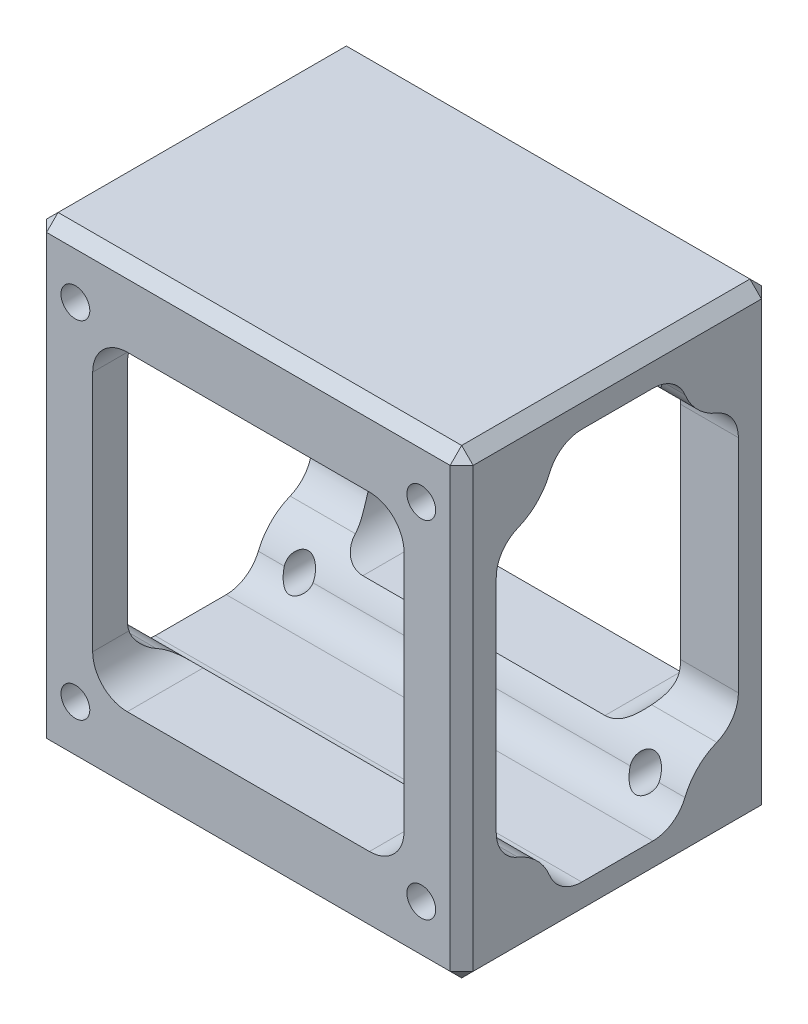
SolidWorks part; units mm, degrees
material "6061 合金"
ref_plane "前视基准面" through (0, 0, 0) normal (0, 0, 1) x (1, 0, 0)
ref_plane "上视基准面" through (0, 0, 0) normal (0, 1, 0) x (1, 0, 0)
ref_plane "右视基准面" through (0, 0, 0) normal (1, 0, 0) x (0, 0, -1)
other "Configuration Table"
sketch "草图1" plane through (0, 0, 0) normal (0, 1, 0) x (1, 0, 0)
  line L1 (-18.5, -13.5) -> (18.5, -13.5)
  line L2 (-18.5, -13.5) -> (-18.5, 13.5)
  line L3 (-18.5, 13.5) -> (18.5, 13.5)
  line L4 (18.5, -13.5) -> (18.5, 13.5)
  line L5 (-18.5, -13.5) -> (18.5, 13.5) construction
  line L6 (-18.5, 13.5) -> (18.5, -13.5) construction
  point P0 (0, 0)
  dimension "D1" = 27
  dimension "D2" = 37
extrude "凸台-拉伸1" add sketch "草图1" along normal blind 40
sketch "草图2" plane through (0, 40, 0) normal (0, 1, 0) x (1, 0, 0)
  line L1 (-10.5, -8.5) -> (10.5, -8.5)
  line L2 (-13.5, -5.5) -> (-13.5, 5.5)
  line L3 (-10.5, 8.5) -> (10.5, 8.5)
  line L4 (13.5, -5.5) -> (13.5, 5.5)
  line L5 (-13.5, -8.5) -> (13.5, 8.5) construction
  line L6 (-13.5, 8.5) -> (13.5, -8.5) construction
  line L14 (15.5, -10.5) -> (15.5, 10.5)
  line L15 (15.5, 10.5) -> (-15.5, 10.5)
  line L16 (-15.5, 10.5) -> (-15.5, -10.5)
  line L17 (-15.5, -10.5) -> (15.5, -10.5)
  line L18 (15.5, -10.5) -> (15.5, 10.5) construction
  line L19 (15.5, 10.5) -> (-15.5, 10.5) construction
  line L20 (-15.5, 10.5) -> (-15.5, -10.5) construction
  line L21 (-15.5, -10.5) -> (15.5, -10.5) construction
  arc A0 (10.5, -8.5) -> (13.5, -5.5) centre (10.5, -5.5) ccw
  arc A1 (-13.5, 5.5) -> (-10.5, 8.5) centre (-10.5, 5.5) cw
  arc A2 (-10.5, -8.5) -> (-13.5, -5.5) centre (-10.5, -5.5) cw
  arc A3 (10.5, 8.5) -> (13.5, 5.5) centre (10.5, 5.5) cw
  circle A4 centre (-15.5, 10.5) radius 1.25 construction
  circle A5 centre (15.5, 10.5) radius 1.25 construction
  circle A6 centre (15.5, -10.5) radius 1.25 construction
  circle A7 centre (-15.5, -10.5) radius 1.25 construction
  point P0 (0, 0)
  dimension "D1" = 17
  dimension "D3" = 3
  dimension "D5" = 2.5
  dimension "D2" = 27
  dimension "D4" = 3
extrude "切除-拉伸2" [suppressed] cut sketch "草图2" against normal through all
sketch "草图3" plane through (0, 0, -13.5) normal (0, 0, -1) x (-1, 0, 0)
  line L4 (18.5, 40) -> (18.5, 0) construction
  line L5 (-15, 5) -> (15, 5) construction
  line L6 (-15, 5) -> (-15, 35) construction
  line L7 (-15, 35) -> (15, 35) construction
  line L8 (15, 5) -> (15, 35) construction
  line L9 (18.5, 40) -> (18.5, 0) construction
  line L10 (-10.5, 6.5) -> (10.5, 6.5)
  line L11 (13.5, 9.5) -> (13.5, 30.5)
  line L12 (-10.5, 33.5) -> (10.5, 33.5)
  line L13 (-13.5, 9.5) -> (-13.5, 30.5)
  line L15 (-13.5, 33.5) -> (13.5, 33.5) construction
  line L16 (-13.5, 6.5) -> (-13.5, 33.5) construction
  line L17 (13.5, 6.5) -> (13.5, 33.5) construction
  line L18 (-13.5, 6.5) -> (13.5, 6.5) construction
  circle A0 centre (-15, 35) radius 1.25
  circle A1 centre (15, 35) radius 1.25
  circle A2 centre (-15, 5) radius 1.25
  circle A3 centre (15, 5) radius 1.25
  arc A4 (-10.5, 33.5) -> (-13.5, 30.5) centre (-10.5, 30.5) ccw
  arc A5 (13.5, 30.5) -> (10.5, 33.5) centre (10.5, 30.5) ccw
  arc A6 (10.5, 6.5) -> (13.5, 9.5) centre (10.5, 9.5) ccw
  arc A7 (-10.5, 6.5) -> (-13.5, 9.5) centre (-10.5, 9.5) cw
  point P4 (0, 5)
  point P7 (18.5, 20)
  point P8 (15, 20)
  dimension "D2" = 2.5
  dimension "D4" = 3
  dimension "D1" = 30
  dimension "D3" = 1.5
extrude "切除-拉伸3" cut sketch "草图3" against normal through all
hole_wizard "M3 螺纹孔1" positions "3D草图1" profile "草图6" tap size "M3" standard "GB" end condition through all
sketch3d "3D草图1"
  line L0 (-15, 5, 13.5) -> (-15, 5, -13.5) construction
  line L1 (-15, 35, 13.5) -> (-15, 35, -13.5) construction
  line L2 (15, 35, 13.5) -> (15, 35, -13.5) construction
  line L3 (15, 5, 13.5) -> (15, 5, -13.5) construction
  point P0 (-15, 5, -13.5)
  point P4 (-15, 35, -13.5)
  point P8 (15, 35, -13.5)
  point P12 (15, 5, -13.5)
sketch "草图6" plane through (-15, 5, -13.5) normal (1, 0, 0) x (0, 1, 0)
  line L0 (0, 0) -> (0, 27)
  line L1 (0, 27) -> (1.25, 27)
  line L2 (1.25, 27) -> (1.25, 0)
  line L5 (1.25, 0) -> (0, 0)
  line L11 (0, -6.35) -> (0, 107.95) construction
  dimension "通孔螺纹孔钻头直径" = 2.5
  dimension "通孔螺纹孔钻头深度" = 27
cosmetic thread "孔螺纹线1" parameters "D2"=3
cosmetic thread "孔螺纹线2" parameters "D2"=3
cosmetic thread "孔螺纹线3" parameters "D2"=3
cosmetic thread "孔螺纹线4" parameters "D2"=3
sketch "草图7" plane through (-18.5, 0, 0) normal (-1, 0, 0) x (0, 0, 1)
  line L8 (-10.5, 3) -> (10.5, 3)
  line L9 (10.5, 3) -> (10.5, 37)
  line L10 (10.5, 37) -> (-10.5, 37)
  line L11 (-10.5, 37) -> (-10.5, 3)
  line L12 (-3.0838, 3) -> (3.0838, 3)
  line L13 (10.5, 10.4162) -> (10.5, 29.5838)
  line L14 (3.0838, 37) -> (-3.0838, 37)
  line L15 (-10.5, 29.5838) -> (-10.5, 10.4162)
  arc A1 (-8.625, 32.3649) -> (-5.8649, 35.125) centre (-10.5, 37) ccw
  arc A2 (5.8649, 35.125) -> (8.625, 32.3649) centre (10.5, 37) ccw
  arc A3 (-5.8649, 4.875) -> (-8.625, 7.6351) centre (-10.5, 3) ccw
  arc A4 (8.625, 7.6351) -> (5.8649, 4.875) centre (10.5, 3) ccw
  arc A5 (-5.8649, 4.875) -> (-3.0838, 3) centre (-3.0838, 6) ccw
  arc A6 (8.625, 7.6351) -> (10.5, 10.4162) centre (7.5, 10.4162) ccw
  arc A7 (5.8649, 35.125) -> (3.0838, 37) centre (3.0838, 34) ccw
  arc A8 (-8.625, 32.3649) -> (-10.5, 29.5838) centre (-7.5, 29.5838) ccw
  arc A9 (-5.8649, 35.125) -> (-3.0838, 37) centre (-3.0838, 34) cw
  arc A10 (-8.625, 7.6351) -> (-10.5, 10.4162) centre (-7.5, 10.4162) cw
  arc A11 (5.8649, 4.875) -> (3.0838, 3) centre (3.0838, 6) cw
  arc A12 (8.625, 32.3649) -> (10.5, 29.5838) centre (7.5, 29.5838) cw
  dimension "D1" = 3
  dimension "D2" = 10
  dimension "D3" = 3
extrude "切除-拉伸4" cut sketch "草图7" against normal through all
chamfer "倒角1" distance 1 angle 45 12 edges at (18.5, 0, 0) (0, 0, -13.5) (-18.5, 0, 0) (0, 0, 13.5) (18.5, 40, 0) (18.5, 20, -13.5) (0, 40, -13.5) (18.5, 20, 13.5) (0, 40, 13.5) (-18.5, 20, 13.5) (-18.5, 40, 0) (-18.5, 20, -13.5)
